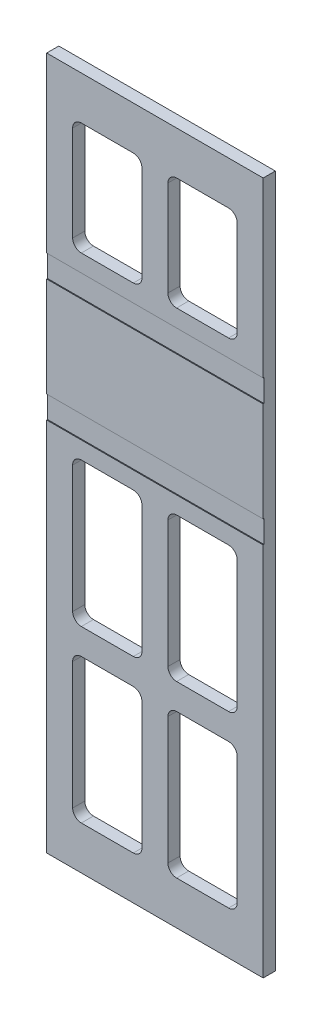
from build123d import *

# Parameters (mm, degrees)
SKETCH_1_W          = 250
SKETCH_1_H          = 800
EXTRUDE_1_DEPTH     = 14
SKETCH_2_W          = 250
SKETCH_2_H          = 26
CUT_EXTRUDE_1_DEPTH = 1
CUT_EXTRUDE_2_REACH = 421.31
SKETCH_3_W          = 80
SKETCH_3_H          = 166.5
SKETCH_3_H_2        = 130
FILLET_1_R          = 10


with BuildPart() as part:
    # 草图1 → 凸台-拉伸1 (new body)
    with BuildSketch(Plane.XY):
        Rectangle(SKETCH_1_W, SKETCH_1_H)
    extrude(amount=EXTRUDE_1_DEPTH)

    # 草图2 → 切除-拉伸1 (cut)
    with BuildSketch(Plane.XY.offset(14)):
        with Locations((0, 187)):
            Rectangle(SKETCH_2_W, SKETCH_2_H)
        with Locations((0, 46)):
            Rectangle(SKETCH_2_W, SKETCH_2_H)
    extrude(amount=-CUT_EXTRUDE_1_DEPTH, mode=Mode.SUBTRACT)

    # 草图3 → 切除-拉伸2 (cut, up to next)
    with BuildSketch(Plane.XY.offset(14), mode=Mode.PRIVATE) as cut_extrude_2_sk1:
        with Locations((-55, -70.25)):
            Rectangle(SKETCH_3_W, SKETCH_3_H)
    cut_extrude_2_tool1 = extrude(cut_extrude_2_sk1.sketch, amount=-CUT_EXTRUDE_2_REACH, mode=Mode.PRIVATE) & part.part
    # 草图3 → 切除-拉伸2 (cut, up to next)
    with BuildSketch(Plane.XY.offset(14), mode=Mode.PRIVATE) as cut_extrude_2_sk2:
        with Locations((-55, -266.75)):
            Rectangle(SKETCH_3_W, SKETCH_3_H)
    cut_extrude_2_tool2 = extrude(cut_extrude_2_sk2.sketch, amount=-CUT_EXTRUDE_2_REACH, mode=Mode.PRIVATE) & part.part
    # 草图3 → 切除-拉伸2 (cut, up to next)
    with BuildSketch(Plane.XY.offset(14), mode=Mode.PRIVATE) as cut_extrude_2_sk3:
        with Locations((55, -266.75)):
            Rectangle(SKETCH_3_W, SKETCH_3_H)
    cut_extrude_2_tool3 = extrude(cut_extrude_2_sk3.sketch, amount=-CUT_EXTRUDE_2_REACH, mode=Mode.PRIVATE) & part.part
    # 草图3 → 切除-拉伸2 (cut, up to next)
    with BuildSketch(Plane.XY.offset(14), mode=Mode.PRIVATE) as cut_extrude_2_sk4:
        with Locations((55, -70.25)):
            Rectangle(SKETCH_3_W, SKETCH_3_H)
    cut_extrude_2_tool4 = extrude(cut_extrude_2_sk4.sketch, amount=-CUT_EXTRUDE_2_REACH, mode=Mode.PRIVATE) & part.part
    # 草图3 → 切除-拉伸2 (cut, up to next)
    with BuildSketch(Plane.XY.offset(14), mode=Mode.PRIVATE) as cut_extrude_2_sk5:
        with Locations((-55, 285)):
            Rectangle(SKETCH_3_W, SKETCH_3_H_2)
    cut_extrude_2_tool5 = extrude(cut_extrude_2_sk5.sketch, amount=-CUT_EXTRUDE_2_REACH, mode=Mode.PRIVATE) & part.part
    # 草图3 → 切除-拉伸2 (cut, up to next)
    with BuildSketch(Plane.XY.offset(14), mode=Mode.PRIVATE) as cut_extrude_2_sk6:
        with Locations((55, 285)):
            Rectangle(SKETCH_3_W, SKETCH_3_H_2)
    cut_extrude_2_tool6 = extrude(cut_extrude_2_sk6.sketch, amount=-CUT_EXTRUDE_2_REACH, mode=Mode.PRIVATE) & part.part
    add(cut_extrude_2_tool1.solids().sort_by_distance((-55, -70.25, 14))[0], mode=Mode.SUBTRACT)
    add(cut_extrude_2_tool2.solids().sort_by_distance((-55, -266.75, 14))[0], mode=Mode.SUBTRACT)
    add(cut_extrude_2_tool3.solids().sort_by_distance((55, -266.75, 14))[0], mode=Mode.SUBTRACT)
    add(cut_extrude_2_tool4.solids().sort_by_distance((55, -70.25, 14))[0], mode=Mode.SUBTRACT)
    add(cut_extrude_2_tool5.solids().sort_by_distance((-55, 285, 14))[0], mode=Mode.SUBTRACT)
    add(cut_extrude_2_tool6.solids().sort_by_distance((55, 285, 14))[0], mode=Mode.SUBTRACT)

    # 圆角1
    fillet_1_edges = [part.edges().sort_by_distance(p)[0] for p in [
        (-15, -183.5, 7),
        (-15, -350, 7),
        (-95, -350, 7),
        (-95, -183.5, 7),
        (95, -183.5, 7),
        (95, -350, 7),
        (15, -350, 7),
        (15, -183.5, 7),
        (95, 13, 7),
        (95, -153.5, 7),
        (15, -153.5, 7),
        (15, 13, 7),
        (-15, 350, 7),
        (-15, 220, 7),
        (-95, 220, 7),
        (-95, 350, 7),
        (95, 350, 7),
        (95, 220, 7),
        (15, 220, 7),
        (15, 350, 7),
        (-15, 13, 7),
        (-15, -153.5, 7),
        (-95, -153.5, 7),
        (-95, 13, 7),
    ]]
    fillet(fillet_1_edges, radius=FILLET_1_R)


solid = part.part
